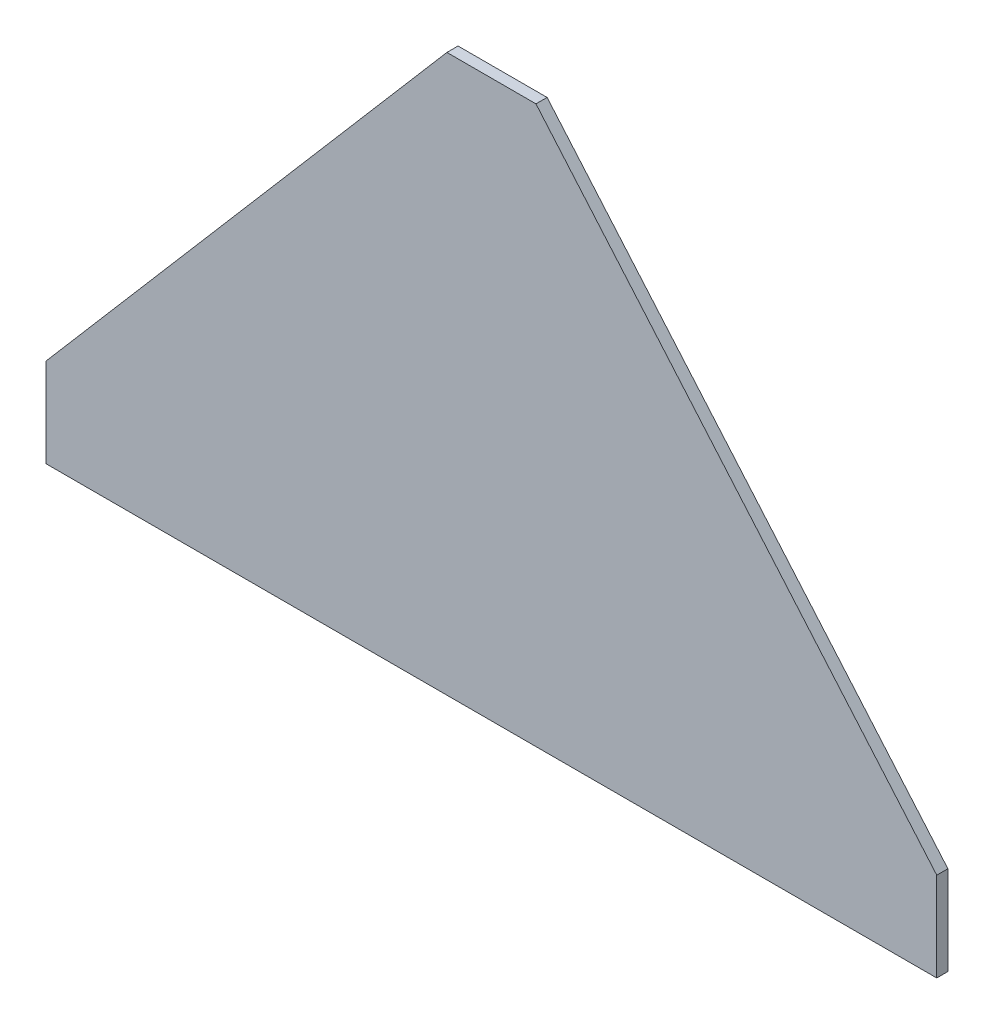
SolidWorks part; units mm, degrees
material "1023 碳钢板 (SS)"
ref_plane "Front Plane" through (0, 0, 0) normal (0, 0, 1) x (1, 0, 0)
ref_plane "Top Plane" through (0, 0, 0) normal (0, 1, 0) x (1, 0, 0)
ref_plane "Right Plane" through (0, 0, 0) normal (1, 0, 0) x (0, 0, -1)
sketch "Sketch1" plane through (0, 0, 0) normal (0, 0, 1) x (1, 0, 0)
  line L1 (200, 125) -> (-200, 125)
  line L2 (200, 125) -> (200, -125)
  line L3 (200, -125) -> (-200, -125)
  line L4 (-200, 125) -> (-200, -125)
  line L5 (200, 125) -> (-200, -125) construction
  line L6 (200, -125) -> (-200, 125) construction
  point P0 (0, 0)
  dimension "D1" = 400
  dimension "D2" = 250
extrude "Boss-Extrude1" add sketch "Sketch1" along normal blind 5
sketch "Sketch2" plane through (0, 0, 5) normal (0, 0, 1) x (1, 0, 0)
  line L0 (-200, -85) -> (-20, 125)
  line L1 (-200, 125) -> (-200, -125) construction
  line L2 (200, 125) -> (-200, 125) construction
  line L3 (-20, 125) -> (20, 125)
  line L4 (20, 125) -> (200, -85)
  line L5 (200, -125) -> (200, 125) construction
  line L7 (-200, -85) -> (-200, -125)
  line L8 (-200, -125) -> (200, -125)
  line L9 (200, -125) -> (200, -85)
  dimension "D1" = 210
  dimension "D2" = 40
extrude "Cut-Extrude1" cut sketch "Sketch2" against normal blind 5 flip side to cut
